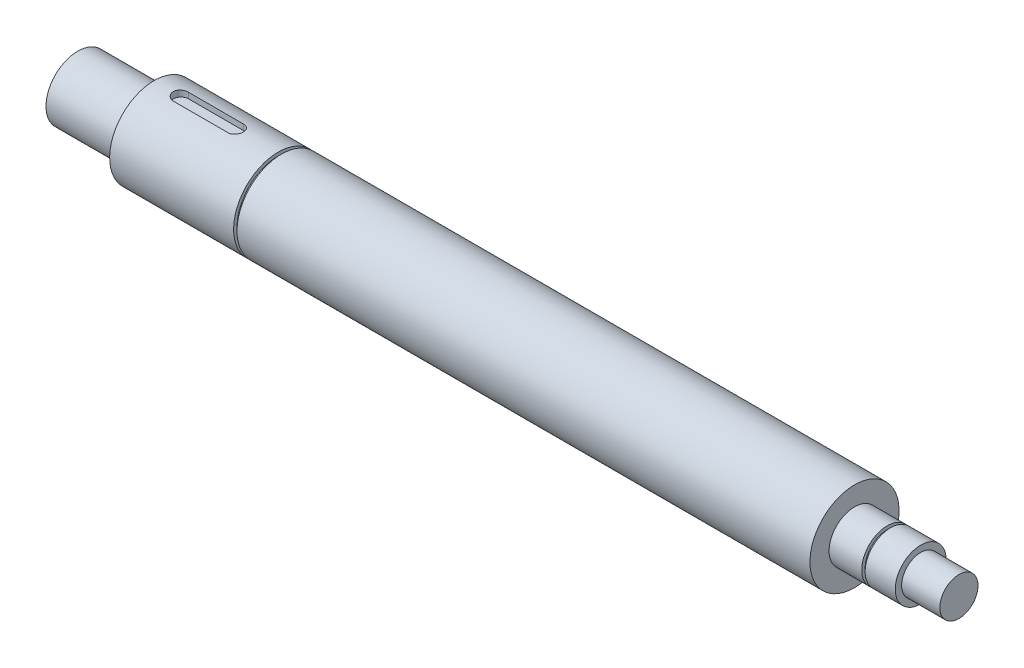
from build123d import *

# Parameters (mm, degrees)
CUT_EXTRUDE1_DEPTH      = 1
CUT_EXTRUDE1_DEPTH_BACK = 35
CUT_EXTRUDE1_START      = 65


with BuildPart() as part:
    # Sketch1 → Revolve1 (revolve)
    with BuildSketch(Plane.XY, mode=Mode.PRIVATE) as revolve1_sk:
        Polygon((0, 0), (0, 25), (60, 25), (60, 35), (157.35, 35), (157.35, 32.35), (160, 32.35), (160, 35), (610, 35), (610, 20), (635.67, 20), (635.67, 17.35), (638.32, 17.35), (638.32, 20), (661.99, 20), (661.99, 15), (691.99, 15), (691.99, 0), align=None)
    revolve(revolve1_sk.sketch.rotate(Axis((0, 0, 0), (1, 0, 0)), 180), axis=Axis((0, 0, 0), (1, 0, 0)))

    # Sketch2 → Cut-Extrude1 (cut, two sides: drawn at the far end of the back side and taken through both)
    with BuildSketch(Plane(origin=(0, 0, 0), x_dir=(1, 0, 0), z_dir=(0, 1, 0)).offset(CUT_EXTRUDE1_START - CUT_EXTRUDE1_DEPTH_BACK)):
        with BuildLine():
            Line((81, 6), (124, 6))
            ThreePointArc((124, 6), (130, 0), (124, -6))
            Line((124, -6), (81, -6))
            ThreePointArc((81, -6), (75, 0), (81, 6))
        make_face()
    extrude(amount=CUT_EXTRUDE1_DEPTH + CUT_EXTRUDE1_DEPTH_BACK, mode=Mode.SUBTRACT)


solid = part.part
